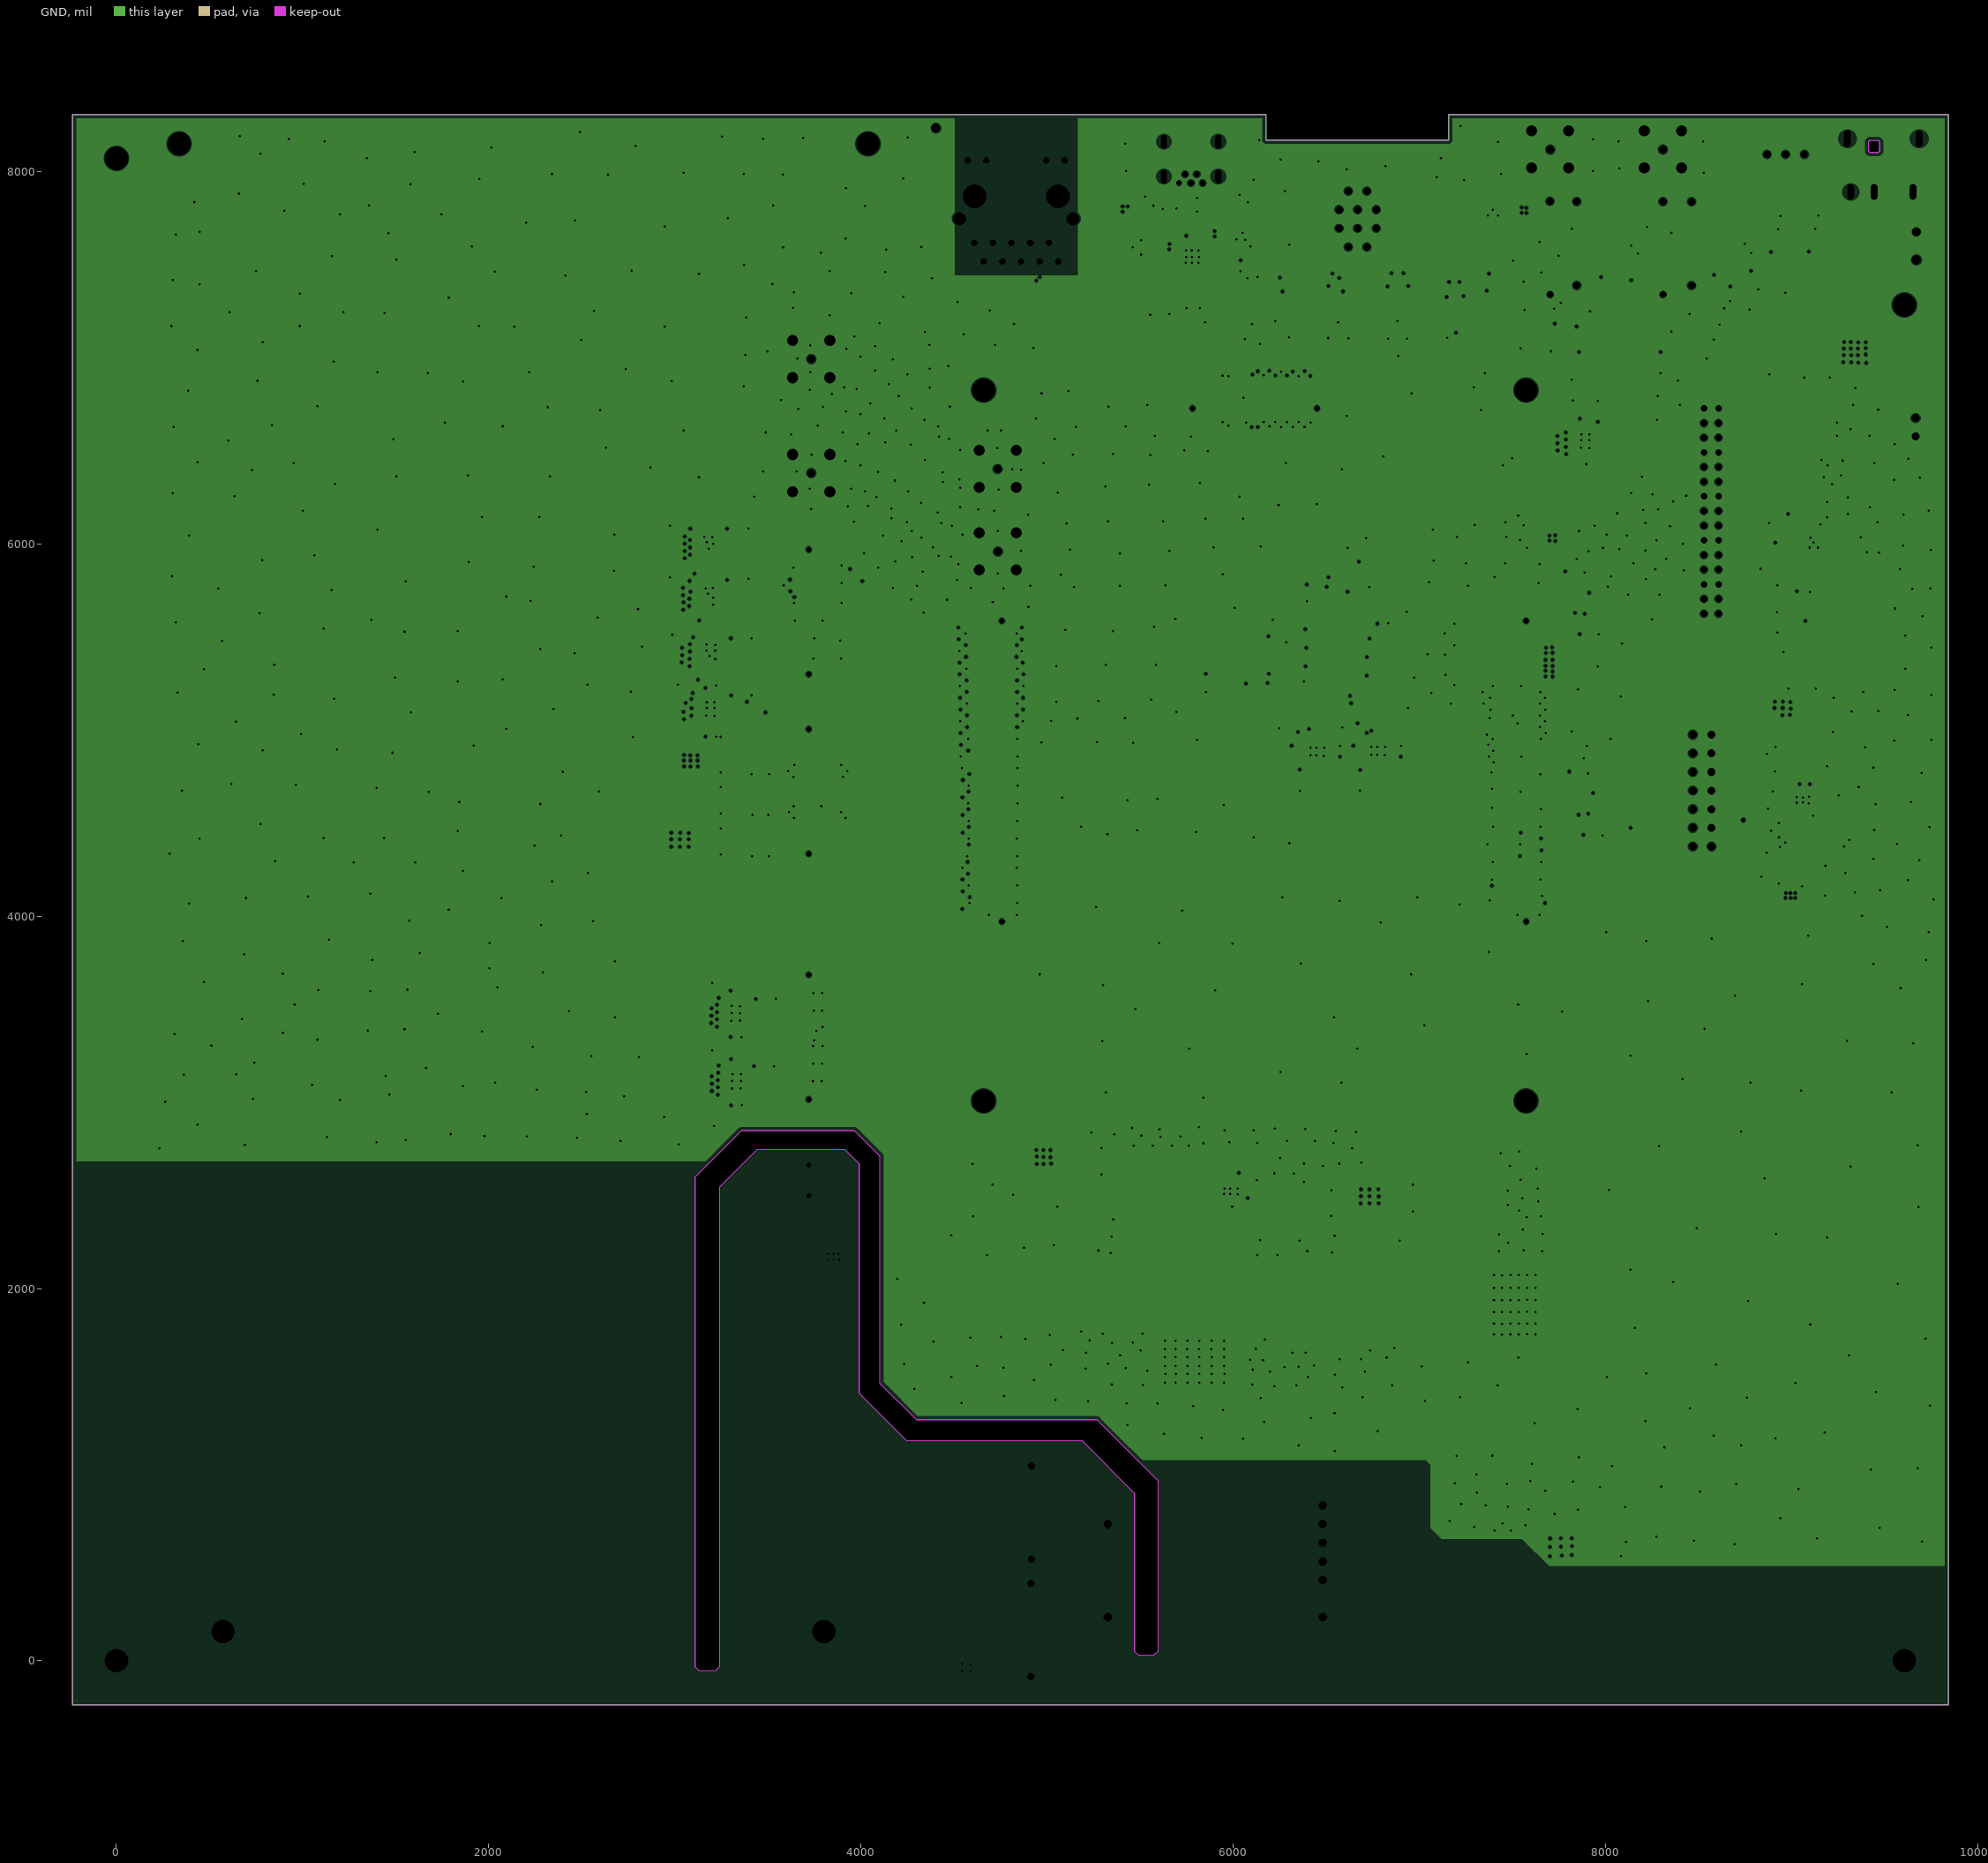
[diagram p0: GND, clearances drawn from the general rule]
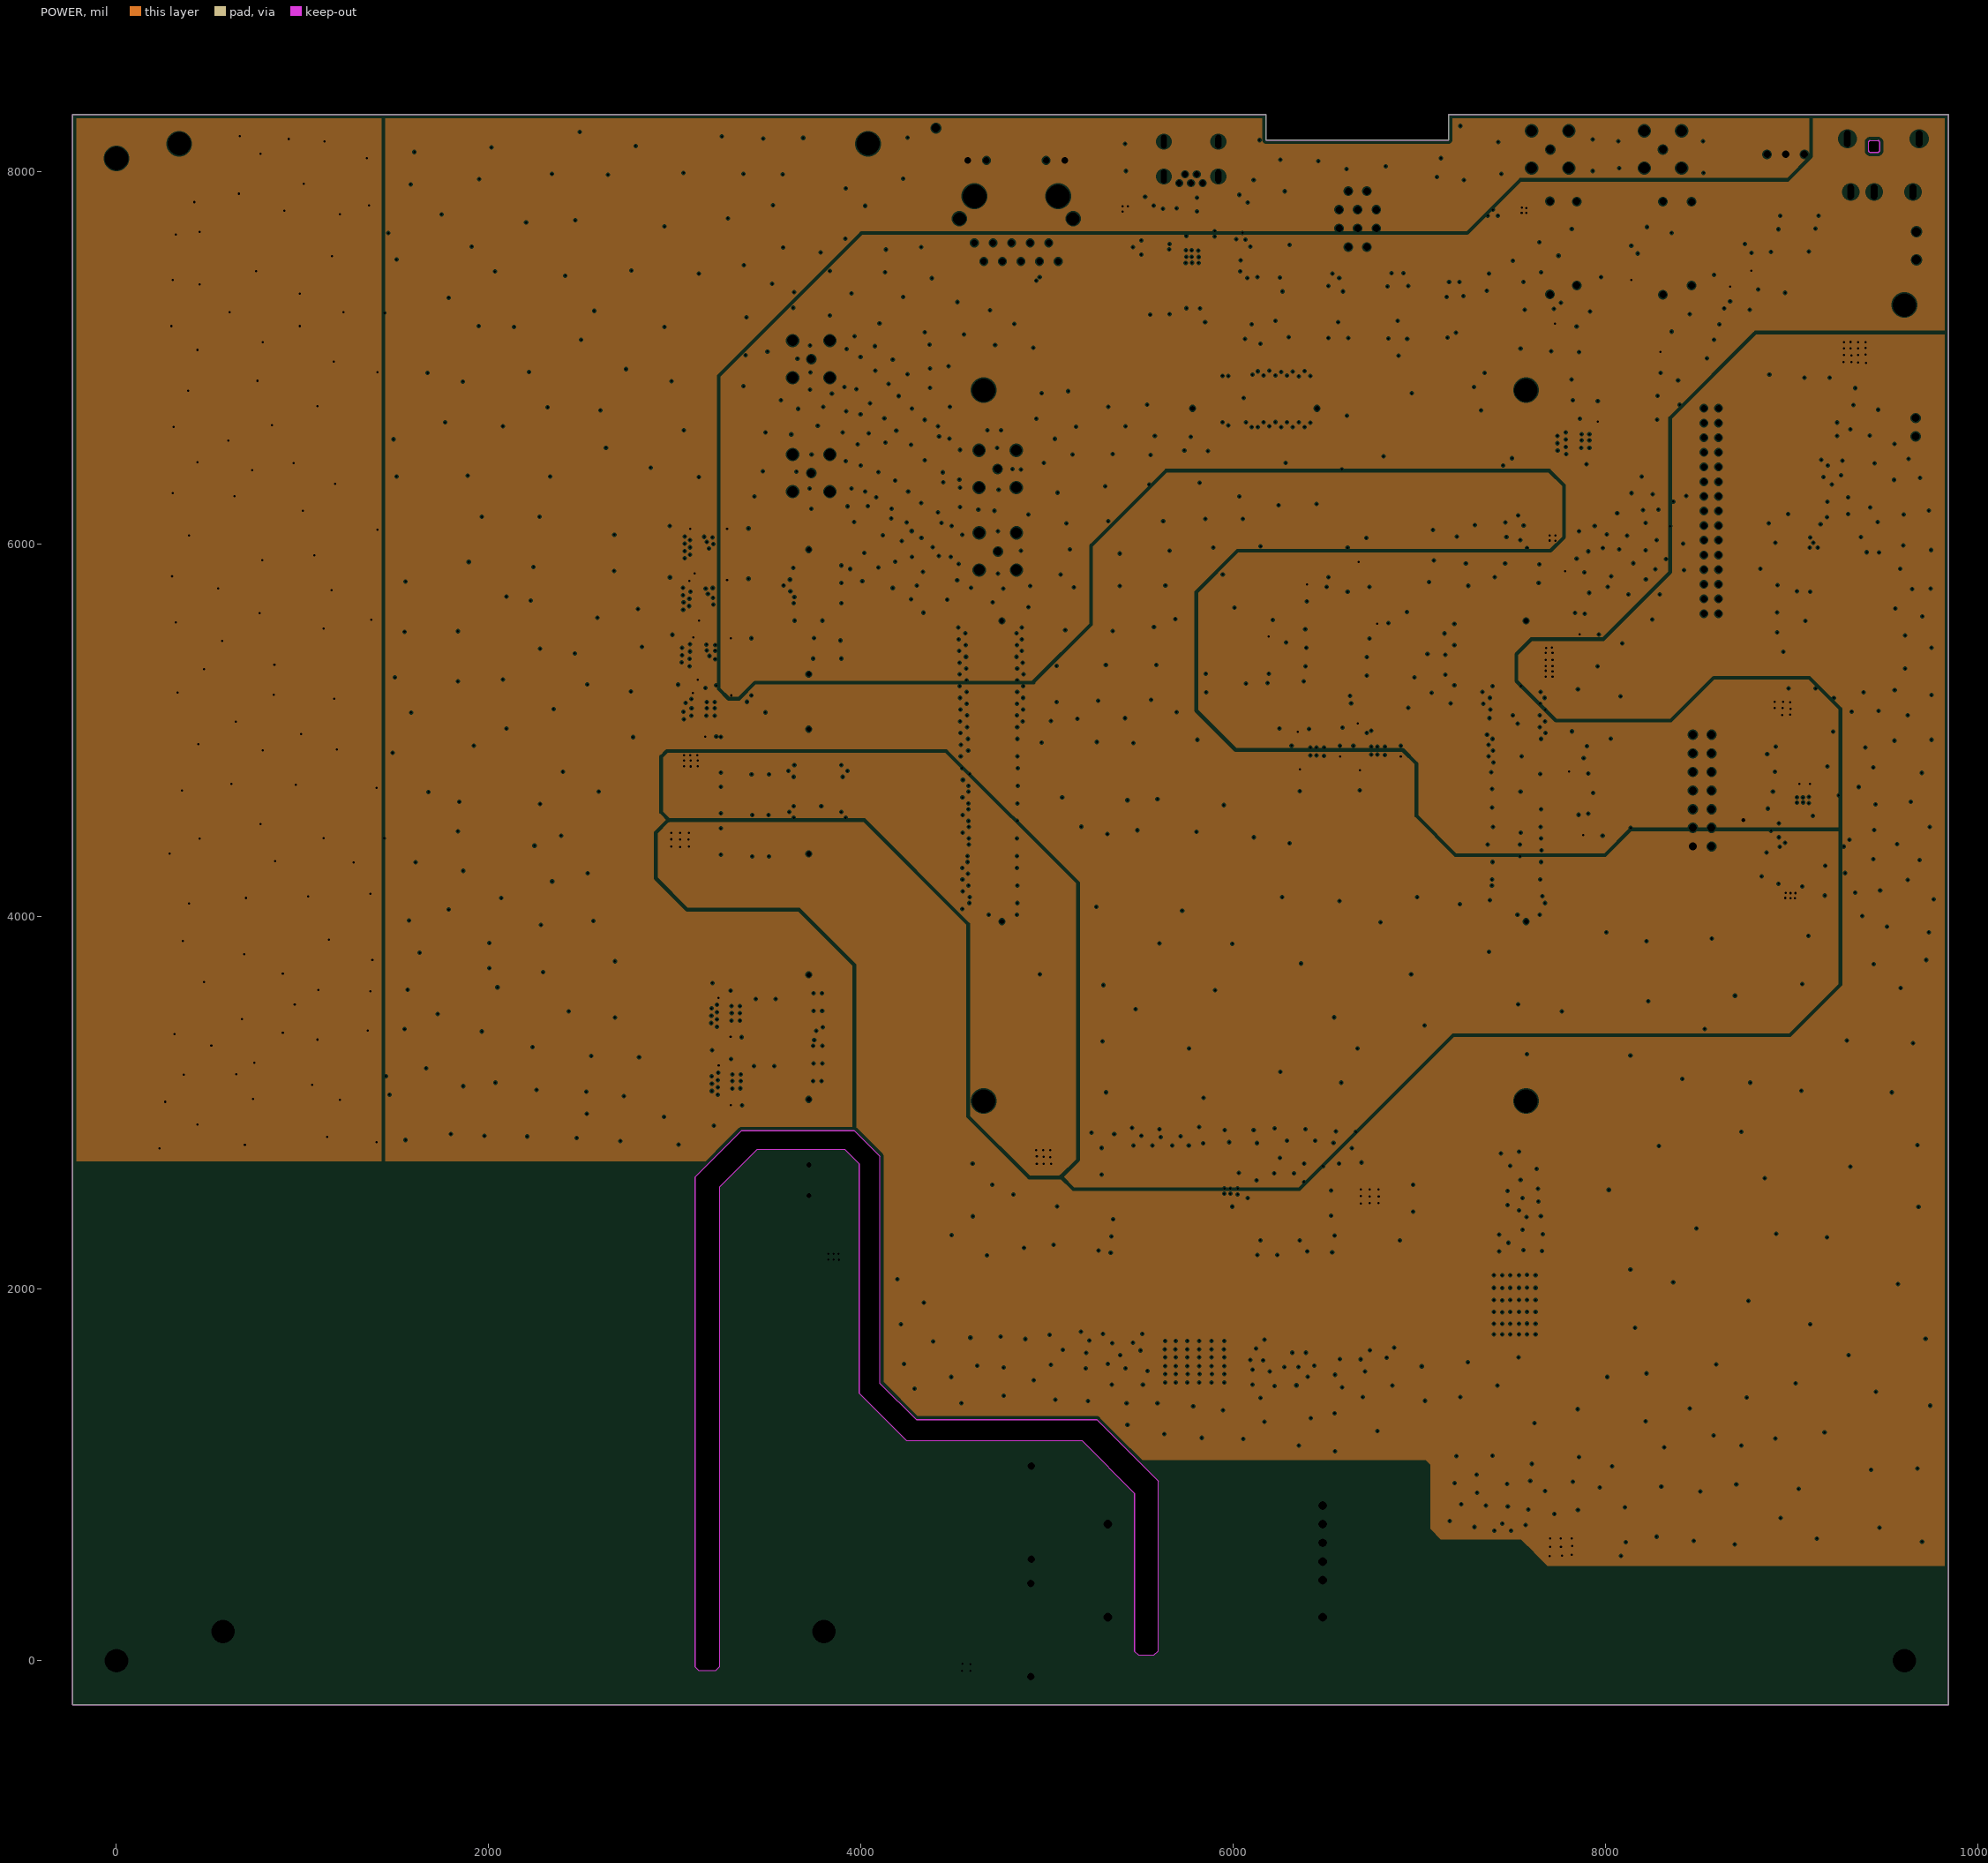
[diagram p1: POWER, clearances drawn from the general rule]
# Altium PCB MISC82191.PcbDoc (part 2 of 9)
## Components (designator, comment, footprint, x,y, rotation, side; value= is the part's Value field where it differs from the comment) (continued)
Q3 "MMBT3906/2A" SOT-23 7976.78,7755.16 r0 top
Q4 "MMBT3906/2A" SOT-23 8584.78,7753.16 r0 top
R1 "10K 1%" 0603#1 9280.78,4440.16 r180 top
R2 "35.7K 1%" 0603#1 9028.78,5809.16 r180 top
R3 "31.3K 1%" 0603#1 9135.78,4441.16 r0 top
R4 "56K 1%" 0603#1 8942.78,6036.16 r270 top
R5 "8.06K 1%" 0603#1 9099.78,5808.16 r0 top
R6 "0R1%" 0805#1 9576.52,6879.09 r0 top
R7 "10K 1%" 0603#1 8942.78,6111.16 r270 top
R8 "80.6K 1%" 0603#1 9303.78,6036.16 r90 top
R9 "1.69K 1%" 0603#1 8942.78,5957.16 r270 top
R12 "100K 1%" 0603#1 6056.59,2714.83 r0 top
R13 "143K 1%" 0603#1 5948.59,2682.83 r90 top
R14 "24K 1%" 0603#1 5948.59,2753.83 r90 top
R19 "100R 5%" 0603A 9068.33,7933.36 r180 top
R20 "100R 5%" 0603A 8868.33,7929.36 r180 top
R23 "1K" 0402 5929.78,5668.16 r0 top
R25 "2K 5%" 0603A 9092.4,7613.09 r270 top
R26 "2K 5%" 0603A 8889.4,7611.09 r270 top
R27 "2K 5%" 0603A 9091.33,7693.36 r270 top
R28 "2K 5%" 0603A 8890.33,7690.36 r270 top
R34 "1K" 0402 6080.78,5662.16 r180 top
R35 "100R 5%" 0805R 8058.78,7464.16 r0 top
R36 "100R 5%" 0805R 8055.78,7663.16 r180 top
R37 "100R 1% 1/4W" AXIAL-0.45 7845.78,7389.16 r90 top
R38 "49.9R 1% 1/4W" AXIAL-0.5 7701.78,7340.16 r90 top
R39 "100R 5%" 0805R 8668.78,7467.16 r0 top
R40 "100R 5%" 0805R 8663.78,7661.16 r180 top
R41 "100R 1% 1/4W" AXIAL-0.45 8462.78,7388.16 r90 top
R42 "49.9R 1% 1/4W" AXIAL-0.5 8308.78,7339.16 r90 top
R43 "2.2M 5% 1/4W" AXIAL-0.5 4915.59,546.83 r90 top
R44 "2.2M 5% 1/4W" AXIAL-0.5 4913.59,-84.17 r90 top
R45 "100R" 0603#1 5971.78,7344.16 r0 top
R46 "100R" 0603#1 5897.78,7344.16 r0 top
R47 "10K" 0603#1 5556.78,7500.16 r270 top
R48 "10K" 0603#1 5748.78,7343.16 r0 top
RJ1 "HY911130A" HY911130A 5059.78,7517.16 r0 top
RZ1 "0R" 0805R 7445.78,619.78 r90 top
RZ2 "0R" 0805R 3857.78,2244.41 r90 top
TP1 "" TP1 9055.78,5044.16 r270 top
TP2 "" TP1 8995.78,4280.16 r270 top
TP4 "" TP1 5093.78,2682.41 r180 top
U2 "AMS1117S-1.8" SOT-89-3_L4.5-W2.5-P1.50-LS4.2-BR 7560.47,6152.27 r270 top
U3 "#NAME?" VQFN-14_L3.5-W3.5-P0.50-BL-EP_TPS54622RHLT 9186.78,6036.16 r180 top
U5 "L7809CD2T-TR(ST)" TO-263-2_L10.0-W9.1-P5.08-LS15.2-TL 7097.73,2015.59 r0 top
U6 "L7806CD2T-TR(ST)" TO-263-2_L10.0-W9.1-P5.08-LS15.2-TL 5895.59,2022.83 r270 top
U7 "#NAME?" TDFN-12_L3.0-W3.0-P0.50-BL-EP 6036.59,2575.83 r180 top
U8 "BV05C" SOD-323 6650.78,7428.16 r0 top
U9 "BV05C" SOD-323 7422.78,7429.16 r0 top
U10 "BV05C" SOD-323 7263.78,7429.16 r0 top
U11 "BV05C" SOD-323 6331.78,7430.16 r0 top
U12 "BV05C" SOD-323 6483.78,7429.16 r180 top
U13 "SMBJ33CA /33V" DO-214AC(SMA) 7159.78,7714.23 r90 top
U14 "BV05C" SOD-323 7110.78,7429.16 r0 top
U15 "BV05C" SOD-323 6964.78,7429.16 r180 top
U16 "BV05C" SOD-323 6801.78,7428.16 r0 top
U17 "#NAME?" TSSOP-16_L5.0-W4.4-P0.65-LS6.4-BL 6448.78,5871.16 r270 top
U18 "TXB0108RGYR" QFN20 3151.68,6081.78 r270 top
U19 "TXB0108RGYR" QFN20 3163.78,5502.78 r270 top
U20 "TXB0108RGYR" QFN20 6358.8,4856.72 r0 top
U21 "#NAME?" TSSOP-16_L5.0-W4.4-P0.65-LS6.4-BL 7784.78,5568.16 r0 top
U22 "#NAME?" TSSOP-16_L5.0-W4.4-P0.65-LS6.4-BL 7804.78,4492.16 r0 top
U23 "TXB0108RGYR" QFN20 3153.78,5805.78 r270 top
U24 "TXB0108RGYR" QFN20 3163.78,5197.78 r270 top
U25 "TXB0108RGYR" QFN20 6685.8,4856.72 r0 top
U26 "74HC14D" SO-14 5910.78,5503.16 r270 top
U27 "TXB0108RGYR" QFN20 3301.78,3200.78 r270 top
U28 "TXB0108RGYR" QFN20 7861.78,6641.16 r270 top
U29 "TXB0108RGYR" QFN20 3299.78,3565.78 r270 top
U31 "DW-N601-5CN2" DW-N601-5CN2 6481.59,833.83 r180 top
U32 "CP2104" QFN-24_L4.0-W4.0-P0.50-BL-EP2.7 5826.78,7622.16 r180 top
U33 "RCLAMP0522P" DFN-1610-6_L1.6-W1.0-P0.50-BL 5766.78,7813.16 r0 top
U34 "XC6206P182MR" SOT-23-3_L2.9-W1.6-P1.90-LS2.8-BR 6092.78,7634.16 r270 top
U501 "74HC14D" SO-14 6447.66,5541.72 r270 top
U707 "74HC14D" SO-14 8254.78,7248.78 r180 top

## Footprints (in the part's own frame and the unit in brackets; to place one, negate y for a bottom-side part, rotate by r counter-clockwise, add the part's x,y. Pads: shape width x height; smd on the part's side, far side on the other; paste and mask are expansions set on the pad)
2B-10 [mil]
  round 55 / inner round 60 / far side round 60 hole 40: 1(0,0) 2(50,100) 3(50,200) 4(0,300) 5(-100,300) 6(-150,200) 7(-150,100) 8(-100,0) 9(-50,100) 10(-50,200)
  silkscreen extent -346,-43 242,710
0402 [mm]
  rect 0.566x0.54 smd: 1(0.433,0) 2(-0.433,0)
  silkscreen extent -0.94,-0.5 0.94,0.5
0603#1 [mil]
  rect 30x35 smd: 1(0,30) 2(0,-30)
  silkscreen extent -30,-65 30,65
0603#2 [mil]
  rect 55x45 smd: 1(0,0) 2(0,-72)
  silkscreen extent -42,-106 40,34
0603A [mil]
  rect 38x38 smd: 1(0,0) 2(0,-60)
  silkscreen extent -30,-92 32,28
0805#1 [mil]
  rect 60x50 smd: 1(0,0) 2(90,0)
  silkscreen extent -50,-45 140,45
0805#2 [mil]
  rect 50x40 smd: 1(0,0) 2(0,-80)
  silkscreen extent -33,-110 37,33
0805A [mil]
  rect 50x40 smd: 1(0,0) 2(0,-80)
  silkscreen extent -33,-110 37,33
0805R [mil]
  rect 40x50 smd: 1(0,0) 2(80,0)
  silkscreen extent -35,-40 115,41
1005 [mil]
  rect 72x62 smd: 1(0,0) 2(0,-110)
  silkscreen extent -49,-155 46,51
1206 [mil]
  rect 72x62 smd: 1(0,0) 2(0,-110)
  silkscreen extent -27,-65 36,-46
1812 [mil]
  rect 55.38x137.76 smd paste-3937.01 mask+2: 1(0,0) 2(145.94,0)
  silkscreen extent -37,-80 183,80
3225[1210] [mm] "Chip Resistor; Body 3.2 x 2.5 mm (LxW typ)"
  rect 1.6x2.7 smd: 1(-1.4,0) 2(1.4,0)
  silkscreen extent -0.3,-1.25 0.3,1.25
AXIAL-0.5 [mil]
  round 60 hole 40: 1(0,0) 2(500,0)
  silkscreen extent 48,-59 447,61
AXIAL-0.45 [mil]
  round 60 hole 40: 1(0,0) 2(450,0)
  silkscreen extent 50,-46 397,45
C0402 [mil]
  rect 25x20 smd: 1(0,0) 2(50,0)
  silkscreen extent -28,-23 77,22
CAP-SMD-6.3 [mm]
  rect 3x1 smd: 1(-0.333,0.07) 2(5.267,0.07)
  silkscreen extent -0.83,-3.23 5.77,3.37
CAP-SMD_BD10.0-L10.3-W10.3-LS11.0-R-RD [mm]
  rect 4.8x1.8 smd: 1(0,0) 2(-8.79,0)
  silkscreen extent -9.62,-5.23 0.83,5.23
CONN-TH_2P-P2.50_HX25003-2A [mm]
  rect 1.8x1.8 hole 1.1 paste+0 mask+0.05: 1(-1.25,0)
  round 1.8 hole 1.1 paste+0 mask+0.05: 2(1.25,0)
  silkscreen extent -3.75,-3.7 3.75,2.41
CONN-TH_MTE220-30SL [mm]
  rect 1.5x1.5 hole 0.9: 1(0,0)
  round 1.5 hole 0.9: 2(0,2) 3(2,0) 4(2,2) 5(4,0) 6(4,2) 7(6,0) 8(6,2) 9(8,0) 10(8,2) 11(10,0) 12(10,2) 13(12,0) 14(12,2) 15(14,0) 16(14,2) 17(16,0) 18(16,2) 19(18,0) 20(18,2) 21(20,0) 22(20,2) 23(22,0) 24(22,2) 25(24,0) 26(24,2) 27(26,0) 28(26,2) 29(28,0) 30(28,2)
  silkscreen extent -9,-2.1 37,4.1
CONN-TH_WJ15EDGVC-3.81-2P [mm]
  round 2.2 hole 1.25: 1(0,0) 2(3.81,0)
  silkscreen extent -2.35,-4.06 6.1,2.9
DC-IN-TH_DC-044A-A250 [mm]
  oval 3.5x2 hole 0.9 slot 2.1 at 0 deg paste+0 mask+0.05: 1(0,0) 2(0,8.5) 3(0,3.2)
  oval 3.5x2 hole 0.9 slot 2.3 at 0 deg paste+0 mask+0.05: 4(-7.25,9.35) 5(-7.25,-0.45)
  Keep-Out Layer board cut-out: -7,2.652 -7,3.75 -7,3.75 -7,3.79 -6.97,3.863 -6.913,3.92 -6.84,3.95 -6.8,3.95 -6.8,3.95 -5.6,3.95 -5.56,3.95 -5.487,3.919 -5.43,3.863 -5.4,3.789 -5.4,3.75 -5.4,3.75 -5.4,2.652 -5.4,2.612 -5.43,2.538 -5.486,2.482 -5.56,2.452 -5.6,2.452 -5.6,2.452 -6.8,2.452 -6.839,2.452 -6.913,2.482 -6.969,2.538 -7,2.612 -7,2.652 -7,2.652
  Keep-Out Layer region: -7,2.652 -7,3.75 -7,3.75 -6.8,3.95 -5.6,3.95 -5.4,3.75 -5.4,2.652 -5.6,2.452 -6.8,2.452
  Keep-Out Layer lines w0.025: -7,3.75 cw(c-6.8,3.75) -6.8,3.95 -5.6,3.95 cw(c-5.6,3.75) -5.4,3.75 -5.4,2.652 cw(c-5.6,2.652) -5.6,2.452 -6.8,2.452 cw(c-6.8,2.652) -7,2.652 -7,3.75 ; -7,3.75 -7,3.75
  silkscreen extent -10.3,-0.61 1.38,9.55
DFN-8_L3.0-W3.0-P0.65-BL-EP2.3 [mm]
  rect 0.28x0.665 smd: 1(0,0) 2(0.65,0) 3(1.3,0) 4(1.95,0) 5(1.95,3.001) 6(1.3,3.001) 7(0.65,3.001) 8(0,3.001)
  rect 2.45x1.65 smd: 9(0.975,1.568)
  silkscreen extent -0.55,-0.41 2.5,3.09
DFN-1610-6_L1.6-W1.0-P0.50-BL [mm]
  rect 0.2x0.4 smd: 1(0,0) 2(0.5,0) 5(0.5,0.6) 6(0,0.6)
  rect 0.38x0.42 smd: 3(1,-0.02) 4(1,0.62)
  silkscreen extent -0.3,-0.51 1.3,0.8
DIP3B [mil]
  round 60 / inner round 55 / far side round 60 hole 40: 1(0,0) 2(0,-100) 3(0,-200)
  silkscreen extent -36,-229 207,46
DIP-P [mil]
  round 100 hole 60: 1(0,0) 2(0,-200) 3(200,-200) 4(200,0)
  round 70 hole 45: 5(100,-100)
  silkscreen extent -39,-240 240,42
DO-214AC(SMA) [mil]
  rect 80x80 smd: 1(80,0) 2(-80,0)
  Top Layer pour cut-out: -35,58 -34,59 35,59 35,-62 32,-59 -35,-59
  silkscreen extent -157,-60 140,60
DW-N601-5CN2 [mm]
  round 2 hole 1.2: 1(0,0) 2(0,2.54) 3(0,5.08) 4(0,10.16) 5(0,15.24) 6(29.34,15.24) 7(29.34,2.54) 8(0,7.62)
  silkscreen extent -8.81,-3.88 36.19,19.12
FILTER-SMD_4P-L1.0-W0.5-L [mm]
  rect 0.45x0.5 smd: 1(0,0) 3(1.15,0)
  rect 0.3x0.3 smd: 2(0.575,-0.3) 4(0.575,0.3)
  silkscreen extent -0.63,-0.38 1.34,0.38
FILTER-SMD_4P-L3.2-W1.6-L_YFF31HC [mm]
  rect 1.3x1.2 smd: 1(0,0) 3(3.7,0)
  rect 1.4x0.9 smd: 2(1.85,-0.85) 4(1.85,0.85)
  silkscreen extent -1.72,-0.85 4.6,0.85
HY911130A [mil]
  round 60 hole 36: 1(0,0) 2(-50.35,100) 3(-100,0) 4(-150.35,100) 5(-200,0) 6(-250.35,100) 7(-300,0) 8(-350.35,100) 9(-400,0) 10(-450.35,100) 11(35.63,542.92) 12(-64.37,542.92) 13(-385.98,542.92) 14(-485.99,542.92)
  round 98.42 hole 70.87: 15(-530.1,229.92) 16(79.74,229.92)
  round 127.95 hole 127.95 unplated: ""(-450.18,350) ""(-0.18,350)
  silkscreen extent -540,-60 90,785
IDC-TH_14P-P2.54-V-R2-C7-S2.54 [mm]
  rect 1.8x1.8 hole 1.1: 1(0,0)
  round 1.8 hole 1.1: 2(0,2.54) 3(2.54,0) 4(2.54,2.54) 5(5.08,0) 6(5.08,2.54) 7(7.62,0) 8(7.62,2.54) 9(10.16,0) 10(10.16,2.54) 11(12.7,0) 12(12.7,2.54) 13(15.24,0) 14(15.24,2.54)
  silkscreen extent -5.36,-3.23 20.57,5.79
IND-SMD_L7.8-W7.0-A [mm]
  rect 3.5x7 smd: 1(0,0) 2(5.4,0)
  silkscreen extent -1.2,-3.7 6.6,3.7
MINI-USB-TH_USB-MINI-2 [mm]
  oval 1.2x2.4 hole 0.8 slot 1.9 at 90 deg: 0(-2.14,-0.902) 0(-2.14,-5.652) 0(5.3,-0.902) 0(5.3,-5.652)
  oval 1.041x1.2 hole 0.8: 1(0,0) 2(0.8,-1.204) 3(1.6,0)
  round 1.2 hole 0.8: 4(2.4,-1.204) 5(3.2,0)
  silkscreen extent -2.31,-9.25 5.51,0.1
N0.8mm/8Pin-SOCKET [mm]
  round 0.8 hole 0.68: 0(-3.3,0.65) 0(0.9,0.65)
  rect 0.3x1.8 smd: 1(0,0) 2(0,3.8) 3(-0.8,0) 4(-0.8,3.8) 5(-1.6,0) 6(-1.6,3.8) 7(-2.4,0) 8(-2.4,3.8)
  silkscreen extent -4,-0.4 2.2,4
N0.8mm/40Pin-Plug [mm]
  round 0.8 hole 0.68: 0(-0.9,0.65) 0(16.1,0.65)
  rect 0.3x1.8 smd: 1(0,0) 2(0,3.8) 3(0.8,0) 4(0.8,3.8) 5(1.6,0) 6(1.6,3.8) 7(2.4,0) 8(2.4,3.8) 9(3.2,0) 10(3.2,3.8) 11(4,0) 12(4,3.8) 13(4.8,0) 14(4.8,3.8) 15(5.6,0) 16(5.6,3.8) 17(6.4,0) 18(6.4,3.8) 19(7.2,0) 20(7.2,3.8) 21(8,0) 22(8,3.8) 23(8.8,0) 24(8.8,3.8) 25(9.6,0) 26(9.6,3.8) 27(10.4,0) 28(10.4,3.8) 29(11.2,0) 30(11.2,3.8) 31(12,0) 32(12,3.8) 33(12.8,0) 34(12.8,3.8) 35(13.6,0) 36(13.6,3.8) 37(14.4,0) 38(14.4,3.8) 39(15.2,0) 40(15.2,3.8)
  silkscreen extent -2.1,-0.4 16.8,4
QFN20 [mil]
  rect 32x12 smd: 1(0,0) 10(181.1,0) 11(181.1,59.06) 20(0,59.06)
  rect 12x32 smd: 2(21.65,-37.4) 3(41.34,-37.4) 4(61.02,-37.4) 5(80.71,-37.4) 6(100.39,-37.4) 7(120.08,-37.4) 8(139.76,-37.4) 9(159.45,-37.4) 12(159.45,96.46) 13(139.76,96.46) 14(120.08,96.46) 15(100.39,96.46) 16(80.71,96.46) 17(61.02,96.46) 18(41.34,96.46) 19(21.65,96.46)
  rect 120x80 smd: 11(92.15,29.6)
  silkscreen extent -16,-62 183,95
QFN-24_L4.0-W4.0-P0.50-BL-EP2.7 [mm]
  oval 0.28x0.8 smd: 1(0,0) 2(0.5,0) 3(1,0) 4(1.5,0) 5(2,0) 6(2.5,0) 13(2.5,4) 14(2,4) 15(1.5,4) 16(1,4) 17(0.5,4) 18(0.008,4)
  oval 0.8x0.28 smd: 7(3.25,0.75) 8(3.25,1.25) 9(3.25,1.75) 10(3.25,2.25) 11(3.25,2.75) 12(3.25,3.25) 19(-0.75,3.25) 20(-0.75,2.75) 21(-0.75,2.25) 22(-0.75,1.75) 23(-0.75,1.25) 24(-0.75,0.75)
  rect 2.7x2.7 smd: 25(1.262,2)
  silkscreen extent -0.89,-0.8 3.41,4.15
SB1045L [mm]
  rect 1.5x1.2 smd: 1(-4.2,1) 2(-4.2,-1)
  rect 4.8x3.2 smd: 3(0,0)
  silkscreen extent -3.88,-2 1.48,2
SO-14 [mil]
  oval 22.6x80.24 smd: 1(0,0) 2(50,0) 3(100,0) 4(150,0) 5(200,0) 6(250,0) 7(300,0) 8(300,218.04) 9(250,218.04) 10(200,218.04) 11(150,218.04) 12(100,218.04) 13(50,218.04) 14(0,218.04)
  silkscreen extent -35,-6 323,169
SOD323 [mm]
  rect 0.8x0.8 smd: 1(-1.205,0) 2(1.205,0)
  silkscreen extent -0.86,-0.68 0.84,0.72